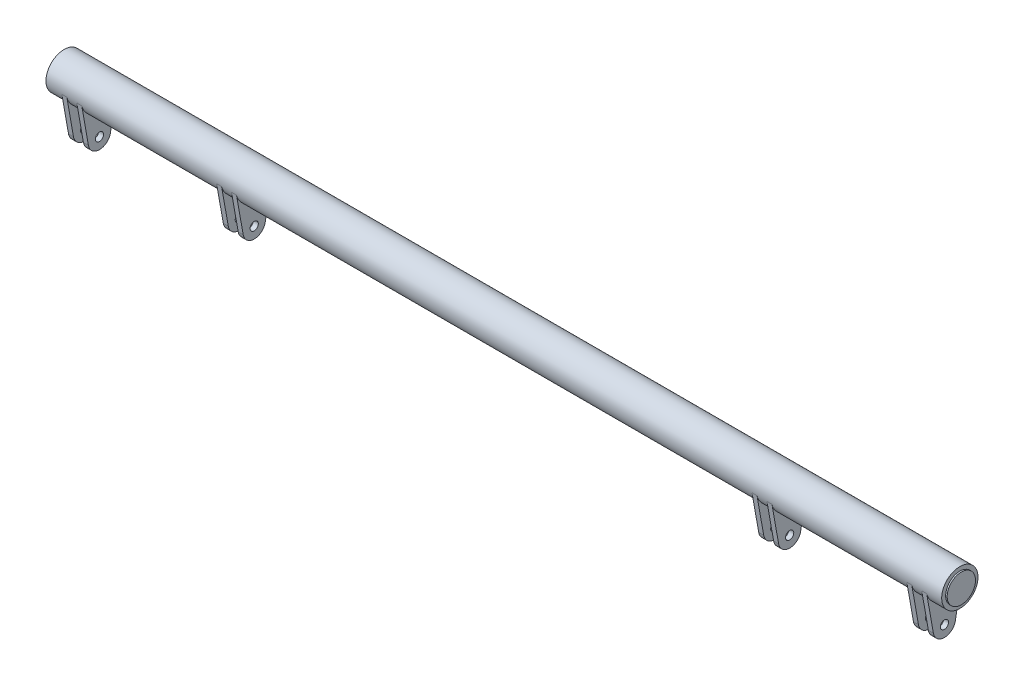
from build123d import *

# Parameters (mm, degrees)
SKETCH1_R                = 36.5
SKETCH1_R_2              = 28.5
STRUCTURAL_MEMBER1_DEPTH = 1800
BOSS_EXTRUDE1_START      = 10
BOSS_EXTRUDE1_DEPTH      = 10
SKETCH4_W                = 8.25
SKETCH4_H                = 10.001
LPATTERN1_COUNT          = 2
LPATTERN1_PITCH          = 30
LPATTERN2_COUNT          = 2
LPATTERN2_PITCH          = 311
SKETCH7_R                = 28.5
BOSS_EXTRUDE2_DEPTH      = 3
SKETCH8_R                = 28.5
BOSS_EXTRUDE3_DEPTH      = 3


with BuildPart() as part:
    # Sketch1 → Structural Member1 (new body)
    with BuildSketch(Plane(origin=(-900, 133.561643836, 0), x_dir=(0, 1, 0), z_dir=(1, 0, 0))):
        Circle(SKETCH1_R)
        Circle(SKETCH1_R_2, mode=Mode.SUBTRACT)
    extrude(amount=STRUCTURAL_MEMBER1_DEPTH)


with BuildPart() as body_2:
    # Sketch3 → Boss-Extrude1 (new body)
    with BuildSketch(Plane(origin=(538, 0, 0), x_dir=(0, 0, -1), z_dir=(1, 0, 0)).offset(BOSS_EXTRUDE1_START)):
        with BuildLine():
            ThreePointArc((35.067814515, 123.239040731), (-1.009482351, 97.020041585), (-35.584230323, 125.190843277))
            Line((-35.584230323, 125.190843277), (-22.152789751, 49.624143836))
            ThreePointArc((-22.152789751, 49.624143836), (-0.62075134, 31.070208404), (21.901886288, 48.408258827))
            Line((21.901886288, 48.408258827), (35.067814515, 123.239040731))
        make_face()
    extrude(amount=BOSS_EXTRUDE1_DEPTH)

    # Sketch4 → Ø16.5 (16.5) Diameter Hole1 (revolve, cut)
    with BuildSketch(Plane(origin=(558, 53.561643836, 0), x_dir=(0, 0, -1), z_dir=(0, 1, 0))):
        with Locations((4.125, 5.0005)):
            Rectangle(SKETCH4_W, SKETCH4_H)
    revolve(axis=Axis((564.35, 53.561643836, 0), (-1, 0, 0)), mode=Mode.SUBTRACT)


with BuildPart() as lpattern1_1:
    # LPattern1: pattern copy
    add(body_2.part.moved(Location(Vector(-1, 0, 0) * (1 * LPATTERN1_PITCH))))


with BuildPart() as body_4:
    # Mirror1: mirrored copy
    add(lpattern1_1.part.mirror(Plane(origin=(0, 0, 0), x_dir=(0, 0, 1), z_dir=(1, 0, 0))))


with BuildPart() as body_5:
    # Mirror1 2: mirrored copy
    add(body_2.part.mirror(Plane(origin=(0, 0, 0), x_dir=(0, 0, 1), z_dir=(1, 0, 0))))


with BuildPart() as lpattern2_1:
    # LPattern2: pattern copy
    add(lpattern1_1.part.moved(Location(Vector(1, 0, 0) * (1 * LPATTERN2_PITCH))))


with BuildPart() as lpattern2_2:
    # LPattern2: pattern copy
    add(body_2.part.moved(Location(Vector(1, 0, 0) * (1 * LPATTERN2_PITCH))))


with BuildPart() as body_8:
    # Mirror2: mirrored copy
    add(lpattern2_1.part.mirror(Plane(origin=(0, 0, 0), x_dir=(0, 0, 1), z_dir=(1, 0, 0))))


with BuildPart() as body_9:
    # Mirror2 2: mirrored copy
    add(lpattern2_2.part.mirror(Plane(origin=(0, 0, 0), x_dir=(0, 0, 1), z_dir=(1, 0, 0))))


with BuildPart() as body_10:
    # Sketch7 → Boss-Extrude2 (new body)
    with BuildSketch(Plane.ZY.offset(900)):
        with Locations((0, 133.561643836)):
            Circle(SKETCH7_R)
    extrude(amount=BOSS_EXTRUDE2_DEPTH)


with BuildPart() as body_11:
    # Sketch8 → Boss-Extrude3 (new body)
    with BuildSketch(Plane(origin=(900, 0, 0), x_dir=(0, 0, -1), z_dir=(1, 0, 0))):
        with Locations((0, 133.561643836)):
            Circle(SKETCH8_R)
    extrude(amount=BOSS_EXTRUDE3_DEPTH)


solid = Compound([part.part, body_2.part, lpattern1_1.part, body_4.part, body_5.part, lpattern2_1.part, lpattern2_2.part, body_8.part, body_9.part, body_10.part, body_11.part])
